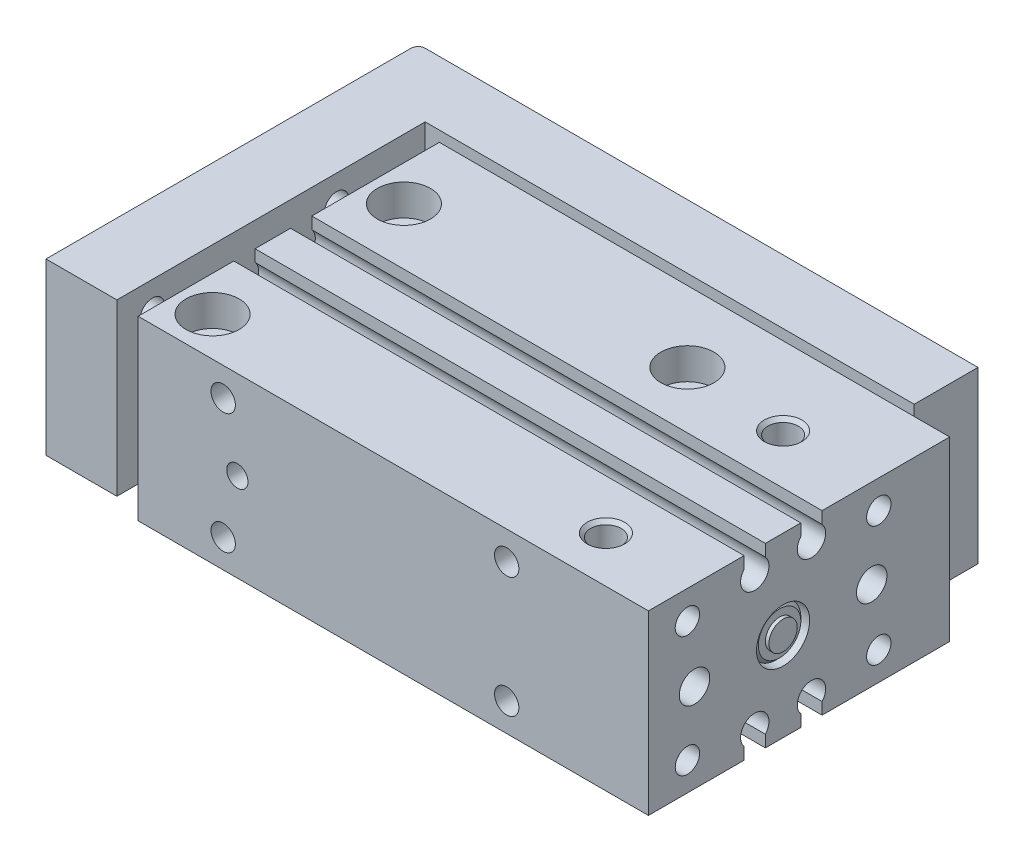
from build123d import *

# Parameters (mm, degrees)
EXTRUDE_1_DEPTH      = 12
SKETCH_3_W           = 72
SKETCH_3_H           = 42.5
EXTRUDE_2_DEPTH      = 12.5
CUT_EXTRUDE_1_DEPTH  = 72
SKETCH_6_R           = 1.72
CUT_EXTRUDE_2_DEPTH  = 6
SKETCH_7_R           = 2.15
CUT_EXTRUDE_3_DEPTH  = 10
SKETCH_8_R           = 2.15
CUT_EXTRUDE_4_DEPTH  = 25
SKETCH_9_R           = 2.15
CUT_EXTRUDE_5_DEPTH  = 4
SKETCH_10_R          = 3.75
CUT_EXTRUDE_6_DEPTH  = 4.4
CHAMFER_2_SIZE       = 0.5
SKETCH_11_R          = 1.72
SKETCH_11_R_2        = 1.5
CUT_EXTRUDE_7_DEPTH  = 6
SKETCH_12_R          = 1.72
SKETCH_12_R_2        = 2.1
CUT_EXTRUDE_8_DEPTH  = 9
SKETCH_14_R          = 1.72
CUT_EXTRUDE_9_DEPTH  = 10
EXTRUDE_3_REACH      = 86.395
SKETCH_16_R          = 2.5
CUT_EXTRUDE_12_DEPTH = 94.501336889
SKETCH_21_R          = 3.75
SKETCH_21_R_2        = 2
EXTRUDE_5_DEPTH      = 5
EXTRUDE_4_DEPTH      = 2
EXTRUDE_4_DEPTH_BACK = 10
SKETCH_17_R          = 2


with BuildPart() as part:
    # 草图2 → 凸台-拉伸1 (new, symmetric)
    with BuildSketch(Plane(origin=(0, 0, 0), x_dir=(1, 0, 0), z_dir=(0, 1, 0))):
        with BuildLine():
            Line((1, 34.5), (79, 34.5))
            Line((79, 34.5), (79, 25.5))
            Line((79, 25.5), (10, 25.5))
            Line((10, 25.5), (10, -18))
            Line((10, -18), (0, -18))
            Line((0, -18), (0, 33.5))
            ThreePointArc((0, 33.5), (0.292893219, 34.207106781), (1, 34.5))
        make_face()
    extrude(amount=EXTRUDE_1_DEPTH, both=True)

    # 草图12 → 切除-拉伸8 (cut)
    with BuildSketch(Plane(origin=(0, 0, -34.5), x_dir=(-1, 0, 0), z_dir=(0, 0, -1))):
        with Locations((-14, -8)):
            Circle(SKETCH_12_R)
        with Locations((-44, -8)):
            Circle(SKETCH_12_R)
        with Locations(Location((-44, 8, 0), (0, 0, 180))):
            Circle(SKETCH_12_R)
        with Locations(Location((-14, 8, 0), (0, 0, 180))):
            Circle(SKETCH_12_R)
        with Locations((-73, 4)):
            Circle(SKETCH_12_R_2)
        with Locations((-65, 4)):
            Circle(SKETCH_12_R_2)
        with Locations(Location((-65, -4, 0), (0, 0, 180))):
            Circle(SKETCH_12_R_2)
        with Locations(Location((-73, -4, 0), (0, 0, 180))):
            Circle(SKETCH_12_R_2)
    extrude(amount=-CUT_EXTRUDE_8_DEPTH, mode=Mode.SUBTRACT)

    # 草图14 → 切除-拉伸9 (cut)
    with BuildSketch(Plane.ZY):
        with Locations((13, -8)):
            Circle(SKETCH_14_R)
        with Locations(Location((13, 8, 0), (0, 0, 180))):
            Circle(SKETCH_14_R)
        with Locations(Location((-13, -8, 0), (0, 0, 180))):
            Circle(SKETCH_14_R)
        with Locations((-13, 8)):
            Circle(SKETCH_14_R)
    extrude(amount=-CUT_EXTRUDE_9_DEPTH, mode=Mode.SUBTRACT)


with BuildPart() as body_2:
    # 草图3 → 凸台-拉伸2 (new, symmetric)
    with BuildSketch(Plane(origin=(0, 0, 0), x_dir=(1, 0, 0), z_dir=(0, 1, 0))):
        with Locations((50, 2.25)):
            Rectangle(SKETCH_3_W, SKETCH_3_H)
    extrude(amount=EXTRUDE_2_DEPTH, both=True)

    # 草图5 → 切除-拉伸1 (cut)
    with BuildSketch(Plane(origin=(86, 0, 0), x_dir=(0, 0, -1), z_dir=(1, 0, 0))):
        with BuildLine():
            Line((-5.5, 10.822875656), (-5.5, 12.5))
            Line((-5.5, 12.5), (-2.5, 12.5))
            Line((-2.5, 12.5), (-2.5, 10.822875656))
            ThreePointArc((-2.5, 10.822875656), (-4, 7.5), (-5.5, 10.822875656))
        make_face()
        with BuildLine():
            Line((-2.5, -10.822875656), (-2.5, -12.5))
            Line((-2.5, -12.5), (-5.5, -12.5))
            Line((-5.5, -12.5), (-5.5, -10.822875656))
            ThreePointArc((-5.5, -10.822875656), (-4, -7.5), (-2.5, -10.822875656))
        make_face()
        with BuildLine():
            Line((5.5, -10.822875656), (5.5, -12.5))
            Line((5.5, -12.5), (2.5, -12.5))
            Line((2.5, -12.5), (2.5, -10.822875656))
            ThreePointArc((2.5, -10.822875656), (4, -7.5), (5.5, -10.822875656))
        make_face()
        with BuildLine():
            Line((2.5, 10.822875656), (2.5, 12.5))
            Line((2.5, 12.5), (5.5, 12.5))
            Line((5.5, 12.5), (5.5, 10.822875656))
            ThreePointArc((5.5, 10.822875656), (4, 7.5), (2.5, 10.822875656))
        make_face()
    extrude(amount=-CUT_EXTRUDE_1_DEPTH, mode=Mode.SUBTRACT)

    # 草图6 → 切除-拉伸2 (cut)
    with BuildSketch(Plane(origin=(86, 0, 0), x_dir=(0, 0, -1), z_dir=(1, 0, 0))):
        with Locations((-13.5, 8.5)):
            Circle(SKETCH_6_R)
        with Locations(Location((-13.5, -8.5, 0), (0, 0, 180))):
            Circle(SKETCH_6_R)
        with Locations((13.5, -8.5)):
            Circle(SKETCH_6_R)
        with Locations(Location((13.5, 8.5, 0), (0, 0, 180))):
            Circle(SKETCH_6_R)
    extrude(amount=-CUT_EXTRUDE_2_DEPTH, mode=Mode.SUBTRACT)

    # 草图7 → 切除-拉伸3 (cut)
    with BuildSketch(Plane(origin=(86, 0, 0), x_dir=(0, 0, -1), z_dir=(1, 0, 0))):
        with Locations((-12.5, 0)):
            Circle(SKETCH_7_R)
        with Locations(Location((12.5, 0, 0), (0, 0, 180))):
            Circle(SKETCH_7_R)
    extrude(amount=-CUT_EXTRUDE_3_DEPTH, mode=Mode.SUBTRACT)

    # 草图8 → 切除-拉伸4 (cut)
    with BuildSketch(Plane(origin=(0, 12.5, 0), x_dir=(1, 0, 0), z_dir=(0, 1, 0))):
        with Locations(Location((19, 13.5, 0), (0, 0, 270))):
            Circle(SKETCH_8_R)
        with Locations(Location((59, 13.5, 0), (0, 0, 270))):
            Circle(SKETCH_8_R)
        with Locations(Location((19, -13.5, 0), (0, 0, 270))):
            Circle(SKETCH_8_R)
    extrude(amount=-CUT_EXTRUDE_4_DEPTH, mode=Mode.SUBTRACT)

    # 草图9 → 切除-拉伸5 (cut)
    with BuildSketch(Plane(origin=(0, 12.5, 0), x_dir=(1, 0, 0), z_dir=(0, 1, 0))):
        with Locations(Location((73.5, 12.5, 0), (0, 0, 270))):
            Circle(SKETCH_9_R)
        with Locations(Location((73.5, -12.5, 0), (0, 0, 90))):
            Circle(SKETCH_9_R)
    cut_extrude_5 = extrude(amount=-CUT_EXTRUDE_5_DEPTH, mode=Mode.SUBTRACT)

    # 草图10 → 切除-拉伸6 (cut)
    with BuildSketch(Plane(origin=(0, 12.5, 0), x_dir=(1, 0, 0), z_dir=(0, 1, 0))):
        with Locations(Location((19, 13.5, 0), (0, 0, 270))):
            Circle(SKETCH_10_R)
        with Locations(Location((59, 13.5, 0), (0, 0, 270))):
            Circle(SKETCH_10_R)
        with Locations(Location((19, -13.5, 0), (0, 0, 270))):
            Circle(SKETCH_10_R)
    cut_extrude_6 = extrude(amount=-CUT_EXTRUDE_6_DEPTH, mode=Mode.SUBTRACT)

    # 镜向1: 切除-拉伸5, 切除-拉伸6 across plane
    add(cut_extrude_5.mirror(Plane.ZX), mode=Mode.SUBTRACT)
    add(cut_extrude_6.mirror(Plane.ZX), mode=Mode.SUBTRACT)

    # 倒角2
    chamfer_2_edges = [body_2.edges().sort_by_distance(p)[0] for p in [
        (73.5, 12.5, -14.65),
        (73.5, 12.5, 14.65),
        (73.5, -12.5, -14.65),
        (73.5, -12.5, 14.65),
    ]]
    chamfer(chamfer_2_edges, length=CHAMFER_2_SIZE)

    # 草图11 → 切除-拉伸7 (cut)
    with BuildSketch(Plane.XY.offset(19)):
        with Locations((26, 8.5)):
            Circle(SKETCH_11_R)
        with Locations((66, 8.5)):
            Circle(SKETCH_11_R)
        with Locations(Location((66, -8.5, 0), (0, 0, 180))):
            Circle(SKETCH_11_R)
        with Locations(Location((26, -8.5, 0), (0, 0, 180))):
            Circle(SKETCH_11_R)
        with Locations((28, 0)):
            Circle(SKETCH_11_R_2)
    extrude(amount=-CUT_EXTRUDE_7_DEPTH, mode=Mode.SUBTRACT)

    # 草图16 → 凸台-拉伸3 (add, up to next)
    with BuildSketch(Plane(origin=(10, 0, 0), x_dir=(0, 0, -1), z_dir=(1, 0, 0)), mode=Mode.PRIVATE) as extrude_3_sk1:
        with Locations(Location((0, 0, 0), (0, 0, 180))):
            Circle(SKETCH_16_R)
    extrude_3_tool1 = extrude(extrude_3_sk1.sketch, amount=EXTRUDE_3_REACH, mode=Mode.PRIVATE) - body_2.part

    add(part.part)  # 凸台-拉伸3 merges part
    add(extrude_3_tool1.solids().sort_by_distance((10, 0, 0))[0])

    # 草图18 → 切除-拉伸12 (cut, through all)
    with BuildSketch(Plane.ZY):
        with BuildLine():
            Line((3, 2.25), (3, -2.25))
            ThreePointArc((3, -2.25), (3.557562368, -1.185854123), (3.75, 0))
            ThreePointArc((3.75, 0), (3.557562368, 1.185854123), (3, 2.25))
        make_face()
        with BuildLine():
            ThreePointArc((-3, 2.25), (-3.75, 0), (-3, -2.25))
            Line((-3, -2.25), (-3, 2.25))
        make_face()
        with BuildLine():
            ThreePointArc((-3, -2.25), (0, -3.75), (3, -2.25))
            Line((3, -2.25), (3, 2.25))
            ThreePointArc((3, 2.25), (0, 3.75), (-3, 2.25))
            Line((-3, 2.25), (-3, -2.25))
        make_face()
    extrude(amount=-CUT_EXTRUDE_12_DEPTH, mode=Mode.SUBTRACT)


with BuildPart() as cut_extrude_12_piece_1:
    # of the separate pieces the step leaves, piece 1, a body of its own (cut_extrude_12_pieces)
    add(body_2.part.solids().sort_by_distance((14, -12.5, 19))[0])


with BuildPart() as cut_extrude_12_piece_2:
    # of the separate pieces the step leaves, piece 2, a body of its own (cut_extrude_12_pieces)
    add(body_2.part.solids().sort_by_distance((0, -12, -33.5))[0])


with BuildPart() as body_3:
    # 草图21 → 凸台-拉伸5 (new body)
    with BuildSketch(Plane(origin=(10, 0, 0), x_dir=(0, 0, -1), z_dir=(1, 0, 0))):
        Circle(SKETCH_21_R)
        Circle(SKETCH_21_R_2, mode=Mode.SUBTRACT)
    extrude(amount=-EXTRUDE_5_DEPTH)


with BuildPart() as body_4:
    # 草图17 → 凸台-拉伸4 (new, two sides: drawn at the far end of the back side and taken through both)
    with BuildSketch(Plane(origin=(10, 0, 0), x_dir=(0, 0, -1), z_dir=(1, 0, 0)).offset(-EXTRUDE_4_DEPTH_BACK)):
        Polygon((3.464101615, 0), (1.732050808, 3), (-1.732050808, 3), (-3.464101615, 0), (-1.732050808, -3), (1.732050808, -3), align=None)
        Circle(SKETCH_17_R, mode=Mode.SUBTRACT)
    extrude(amount=EXTRUDE_4_DEPTH + EXTRUDE_4_DEPTH_BACK)

    # 草图19 → 切除-旋转1 (revolve, cut)
    with BuildSketch(Plane(origin=(0, 0, 0), x_dir=(1, 0, 0), z_dir=(0, 1, 0)), mode=Mode.PRIVATE) as cut_revolve_1_sk:
        Polygon((11.732050808, 3.464101615), (12, 3), (12, 3.464101615), align=None)
        Polygon((0, 3.464101615), (0, 3), (0.267949192, 3.464101615), align=None)
    revolve(cut_revolve_1_sk.sketch.rotate(Axis((20.777211293, 0, 0), (-1, 0, 0)), 180), axis=Axis((20.777211293, 0, 0), (-1, 0, 0)), mode=Mode.SUBTRACT)

    # 草图20 → 旋转1 (revolve)
    with BuildSketch(Plane.XY, mode=Mode.PRIVATE) as revolve_1_sk:
        Polygon((0, 1.5), (0, 0), (86, 0), (86, 2), (85.5, 2), (85.5, 3), (85, 3.5), (14.5, 3.5), (14, 3), (14, 2), (0.5, 2), align=None)
    revolve(revolve_1_sk.sketch.rotate(Axis((0, 0, 0), (1, 0, 0)), 90), axis=Axis((0, 0, 0), (1, 0, 0)))


solid = Compound([cut_extrude_12_piece_1.part, cut_extrude_12_piece_2.part, body_3.part, body_4.part])
